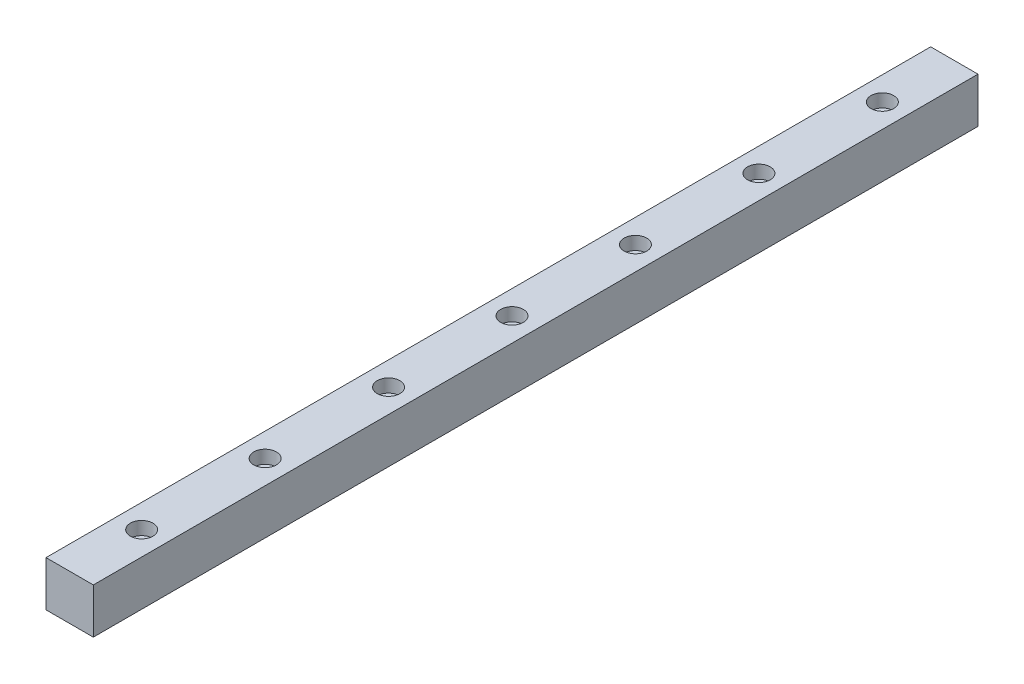
from build123d import *

# Parameters (mm, degrees)
SKETCH_1_W                   = 23
SKETCH_1_H                   = 22
EXTRUDE_1_DEPTH              = 430
HOLE_WIZARD_M6_1_D           = 6.6
HOLE_WIZARD_M6_1_CBORE_D     = 11
HOLE_WIZARD_M6_1_CBORE_DEPTH = 6.4
PATTERN_LINEAR_1_COUNT       = 7
PATTERN_LINEAR_1_PITCH       = 60


with BuildPart() as part:
    # 草图1 → 凸台-拉伸1 (new body)
    with BuildSketch(Plane.XY):
        with Locations((11.5, 11)):
            Rectangle(SKETCH_1_W, SKETCH_1_H)
    extrude(amount=EXTRUDE_1_DEPTH)

    # M6 六角凹头螺钉的柱形沉头孔1 (through all)
    with Locations(Plane(origin=(0, 22, 0), x_dir=(1, 0, 0), z_dir=(0, 1, 0))):
        with Locations((11.5, -395)):
            hole_wizard_m6_1 = CounterBoreHole(HOLE_WIZARD_M6_1_D / 2, HOLE_WIZARD_M6_1_CBORE_D / 2, HOLE_WIZARD_M6_1_CBORE_DEPTH)

    # 阵列(线性)1: M6 六角凹头螺钉的柱形沉头孔1 ×7
    with Locations(*[(0, 0, -i * PATTERN_LINEAR_1_PITCH) for i in range(1, PATTERN_LINEAR_1_COUNT)]):
        add(hole_wizard_m6_1, mode=Mode.SUBTRACT)


solid = part.part
